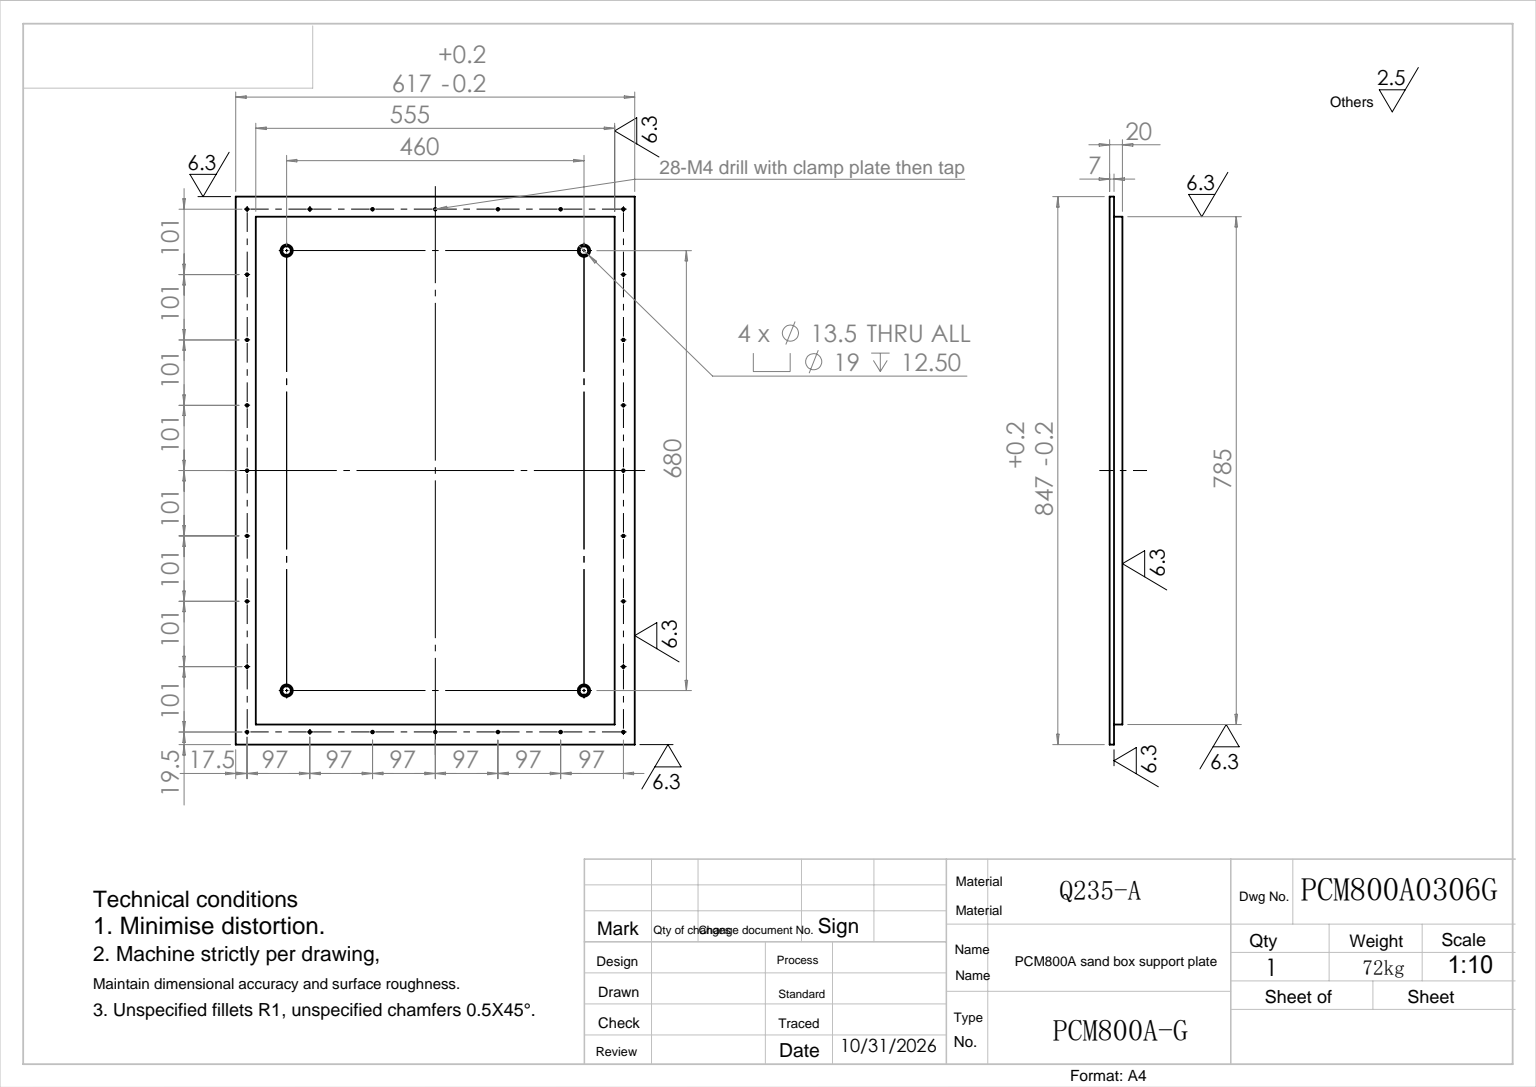
SolidWorks part; units mm, degrees
ref_plane "前视" through (0, 0, 0) normal (0, 0, 1) x (1, 0, 0)
ref_plane "上视" through (0, 0, 0) normal (0, 1, 0) x (1, 0, 0)
ref_plane "右视" through (0, 0, 0) normal (1, 0, 0) x (0, 0, -1)
sketch "草图1" plane through (0, 0, 0) normal (0, 1, 0) x (1, 0, 0)
  line L1 (0, 0) -> (615, 0)
  line L2 (0, 0) -> (0, 845)
  line L3 (0, 845) -> (615, 845)
  line L4 (615, 0) -> (615, 845)
  dimension "D1" = 845
  dimension "D2" = 615
extrude "拉伸1" add sketch "草图1" along normal blind 20
sketch "草图2" plane through (0, 20, 0) normal (0, 1, 0) x (-1, 0, 0)
  line L0 (0, -845) -> (0, 0) construction
  line L1 (-615, -845) -> (0, -845)
  line L2 (-615, -845) -> (-615, -815)
  line L3 (-615, -815) -> (0, -815)
  line L4 (0, -845) -> (0, -815)
  line L6 (-615, 0) -> (0, 0)
  line L7 (-615, 0) -> (-615, -30)
  line L8 (-615, -30) -> (0, -30)
  line L9 (0, 0) -> (0, -30)
  dimension "D1" = 30
  dimension "D2" = 30
extrude "切除-拉伸1" cut sketch "草图2" against normal blind 13
sketch "草图3" plane through (0, 20, 0) normal (0, 1, 0) x (-1, 0, 0)
  line L0 (-615, -30) -> (0, -30) construction
  line L1 (-615, -815) -> (-585, -815)
  line L2 (-615, -815) -> (-615, -30)
  line L3 (-615, -30) -> (-585, -30)
  line L4 (-585, -815) -> (-585, -30)
  line L5 (0, -815) -> (-615, -815) construction
  line L6 (0, -815) -> (-30, -815)
  line L7 (0, -815) -> (0, -30)
  line L8 (0, -30) -> (-30, -30)
  line L9 (-30, -815) -> (-30, -30)
  line L10 (-615, -30) -> (0, -30) construction
  dimension "D1" = 30
  dimension "D2" = 30
  dimension "D3" = 30
extrude "切除-拉伸2" cut sketch "草图3" against normal blind 13
sketch "草图5" plane through (615, 0, 0) normal (1, 0, 0) x (0, 0, -1)
  line L0 (0, 0) -> (845, 0) construction
  line L1 (102.5, 0) -> (372.5, 0)
  line L2 (102.5, 0) -> (102.5, 4.1948)
  line L3 (102.5, 4.1948) -> (372.5, 4.1948)
  line L4 (372.5, 0) -> (372.5, 4.1948)
  line L6 (742.5, 0) -> (472.5, 0)
  line L7 (742.5, 0) -> (742.5, 4.1948)
  line L8 (742.5, 4.1948) -> (472.5, 4.1948)
  line L9 (472.5, 0) -> (472.5, 4.1948)
  dimension "D1" = 270
  dimension "D2" = 102.5
  dimension "D3" = 100
  dimension "D4" = 270
sketch "草图6" plane through (0, 20, 0) normal (0, 1, 0) x (-1, 0, 0)
  line L0 (-307.5, -845) -> (-307.5, 0) construction
  line L1 (-615, -845) -> (0, -845) construction
  line L2 (0, 0) -> (-615, 0) construction
  line L3 (-615, -422.5) -> (0, -422.5) construction
  line L4 (-615, 0) -> (-615, -845) construction
  line L5 (0, -845) -> (0, 0) construction
  line L6 (-545, -762.5) -> (-545, -82.5) construction
  line L7 (-545, -82.5) -> (-70, -82.5) construction
  line L8 (-70, -82.5) -> (-70, -762.5) construction
  line L9 (-70, -762.5) -> (-545, -762.5) construction
  line L10 (-62.5, -622.5) -> (-62.5, -222.5) construction
  dimension "D1" = 340
  dimension "D2" = 340
  dimension "D3" = 237.5
  dimension "D4" = 237.5
  dimension "D5" = 245
  dimension "D6" = 400
  dimension "D7" = 200
sketch "草图8" plane through (0, 20, 0) normal (0, 1, 0) x (-1, 0, 0)
  circle A0 centre (-62.5, -622.5) radius 8
  circle A1 centre (-62.5, -222.5) radius 8
sketch "草图9" plane through (0, 7, 0) normal (0, 1, 0) x (-1, 0, 0)
  line L0 (-598.5, -826.5) -> (-598.5, -18.5) construction
  line L1 (-598.5, -18.5) -> (-16.5, -18.5) construction
  line L2 (-16.5, -18.5) -> (-16.5, -826.5) construction
  line L3 (-16.5, -826.5) -> (-598.5, -826.5) construction
  line L4 (-615, -845) -> (0, -845) construction
  line L5 (-615, 0) -> (-615, -845) construction
  line L6 (0, -845) -> (0, 0) construction
  line L7 (0, 0) -> (-615, 0) construction
  dimension "D1" = 18.5
  dimension "D2" = 16.5
  dimension "D3" = 16.5
  dimension "D4" = 18.5
hole_wizard "M4 螺纹孔1" positions "3D草图2" profile "草图10" tap size "M4" standard "GB" end condition through all
sketch3d "3D草图2"
  point P0 (598.5, 7, -826.5)
  point P3 (16.5, 7, -826.5)
  point P6 (16.5, 7, -18.5)
  point P9 (598.5, 7, -18.5)
sketch "草图10" plane through (598.5, 7, -826.5) normal (1, 0, 0) x (0, 0, 1)
  line L0 (0, 0) -> (0, 7)
  line L1 (0, 7) -> (2, 7)
  line L2 (2, 7) -> (2, 0)
  line L5 (2, 0) -> (0, 0)
  line L11 (0, -6.35) -> (0, 107.95) construction
  dimension "蹟恇盄翋眻噤" = 4
  dimension "籵謂蹟恇謂郰芛旮僅" = 7
pattern_linear "阵列(线性)3" count 8 spacing 101 along (0, 0, 1) of "M4 螺纹孔1"
pattern_linear "阵列(线性)4" count 6 spacing 97 along (-1, 0, 0) of "M4 螺纹孔1"
sketch "草图15" plane through (0, 7, 0) normal (0, 1, 0) x (1, 0, 0)
  line L10 (-1, 846) -> (-1, -1)
  line L11 (-1, -1) -> (616, -1)
  line L12 (616, -1) -> (616, 846)
  line L13 (616, 846) -> (-1, 846)
  line L14 (0, 0) -> (615, 0)
  line L15 (615, 0) -> (615, 845)
  line L16 (0, 845) -> (0, 0)
  line L17 (615, 845) -> (0, 845)
  line L18 (0, 0) -> (615, 0)
  line L19 (615, 0) -> (615, 845)
  line L20 (0, 845) -> (0, 0)
  line L21 (615, 845) -> (0, 845)
  dimension "D1" = 0
  dimension "D2" = 1
extrude "凸台-拉伸5" add sketch "草图15" against normal up to surface (7 mm away) up to face at (113.5, 0, -16.5)
sketch "草图17" plane through (0, 20, 0) normal (0, 1, 0) x (1, 0, 0)
  line L0 (-1, 846) -> (-1, -1) construction
  line L1 (-1, -1) -> (616, -1) construction
  line L2 (616, -1) -> (616, 846) construction
  circle A0 centre (77.5, 82.5) radius 2.5
  circle A1 centre (537.5, 82.5) radius 2.5
  dimension "D3" = 5
  dimension "D6" = 5
  dimension "D1" = 78.5
  dimension "D2" = 83.5
  dimension "D4" = 78.5
  dimension "D5" = 83.5
extrude "切除-拉伸3" cut sketch "草图17" against normal up to surface (20 mm away) up to face at (113.5, 0, -16.5)
hole_wizard "M12 六角头螺栓的柱形沉头孔2" positions "草图20" profile "草图19" counterbore size "M12" standard "Ansi Metric" end condition through all
sketch "草图20" plane through (0, 20, 0) normal (0, 1, 0) x (-1, 0, 0)
  point P0 (-77.5, -82.5)
  point P1 (-537.5, -82.5)
sketch "草图19" plane through (77.5, 20, -82.5) normal (1, 0, 0) x (0, 0, 1)
  line L0 (0, 0) -> (0, 20)
  line L1 (0, 20) -> (6.75, 20)
  line L3 (6.75, 20) -> (6.75, 12.5)
  line L4 (6.75, 12.5) -> (9.5, 12.5)
  line L5 (9.5, 12.5) -> (9.5, 0)
  line L7 (9.5, 0) -> (0, 0)
  line L11 (0, -6.35) -> (0, 107.95) construction
  dimension "通孔孔直径" = 13.5
  dimension "通孔孔深度" = 20
  dimension "柱形沉头孔直径" = 19
  dimension "柱形沉头孔深度" = 12.5
pattern_linear "阵列(线性)7" count 2 spacing 680 along (0, 0, -1) of "M12 六角头螺栓的柱形沉头孔2"
